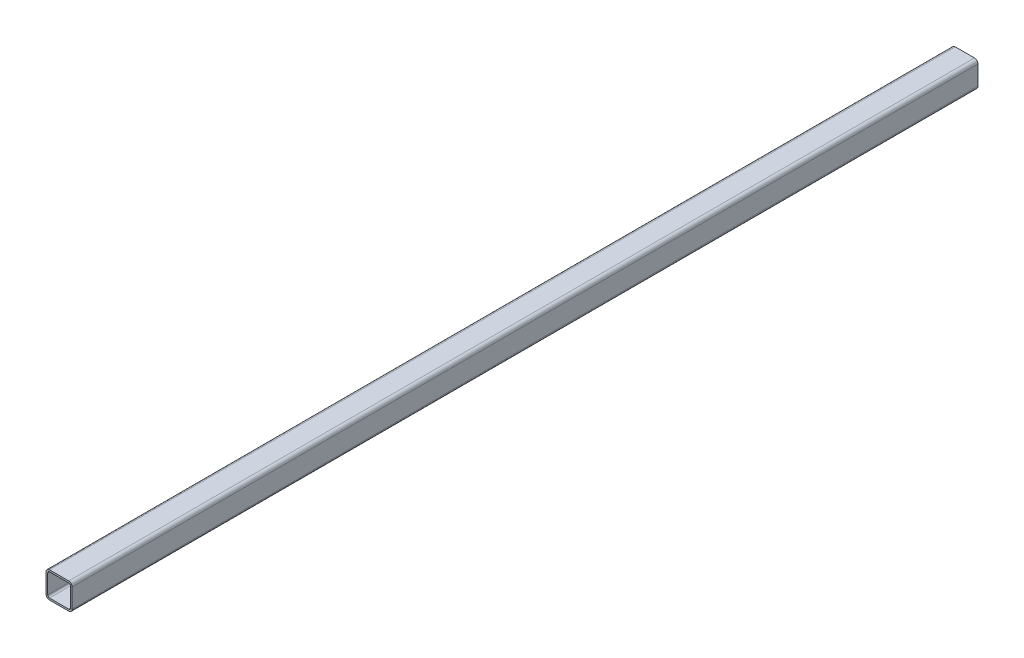
SolidWorks part; units mm, degrees
material "Q235"
ref_plane "Plane1" through (0, 0, 0) normal (0, 0, 1) x (1, 0, 0)
ref_plane "Plane2" through (0, 0, 0) normal (0, 1, 0) x (1, 0, 0)
ref_plane "Plane3" through (0, 0, 0) normal (1, 0, 0) x (0, 0, -1)
sketch "Sketch1" plane through (0, 0, 0) normal (0, 0, 1) x (1, 0, 0)
  line L0 (-11, -13) -> (11, -13)
  line L1 (-13, -11) -> (-13, 11)
  line L2 (11, 13) -> (-11, 13)
  line L3 (13, 11) -> (13, -11)
  line L4 (-11, -15) -> (11, -15)
  line L5 (-15, -11) -> (-15, 11)
  line L6 (11, 15) -> (-11, 15)
  line L7 (15, 11) -> (15, -11)
  arc A0 (15, 11) -> (11, 15) centre (11, 11) ccw
  arc A1 (11, -15) -> (15, -11) centre (11, -11) ccw
  arc A2 (-15, -11) -> (-11, -15) centre (-11, -11) ccw
  arc A3 (-11, 15) -> (-15, 11) centre (-11, 11) ccw
  arc A4 (-11, 13) -> (-13, 11) centre (-11, 11) ccw
  arc A5 (13, 11) -> (11, 13) centre (11, 11) ccw
  arc A6 (11, -13) -> (13, -11) centre (11, -11) ccw
  arc A7 (-13, -11) -> (-11, -13) centre (-11, -11) ccw
  point P0 (-15, 0)
  point P1 (15, 0)
  point P2 (0, 15)
  point P3 (0, -15)
  point P4 (0, 0)
  point P5 (-15, -15)
  point P6 (15, -15)
  point P7 (15, 15)
  point P8 (-15, 15)
  point P33 (0, 5)
  point P35 (-5, 0)
  point P36 (5, 0)
  point P37 (0, -5)
extrude "Extrude-Thin1" add sketch "Sketch1" along normal mid plane 1037.6 thin contours L6 A3 L5 A2 L4 A1 L7 A0
